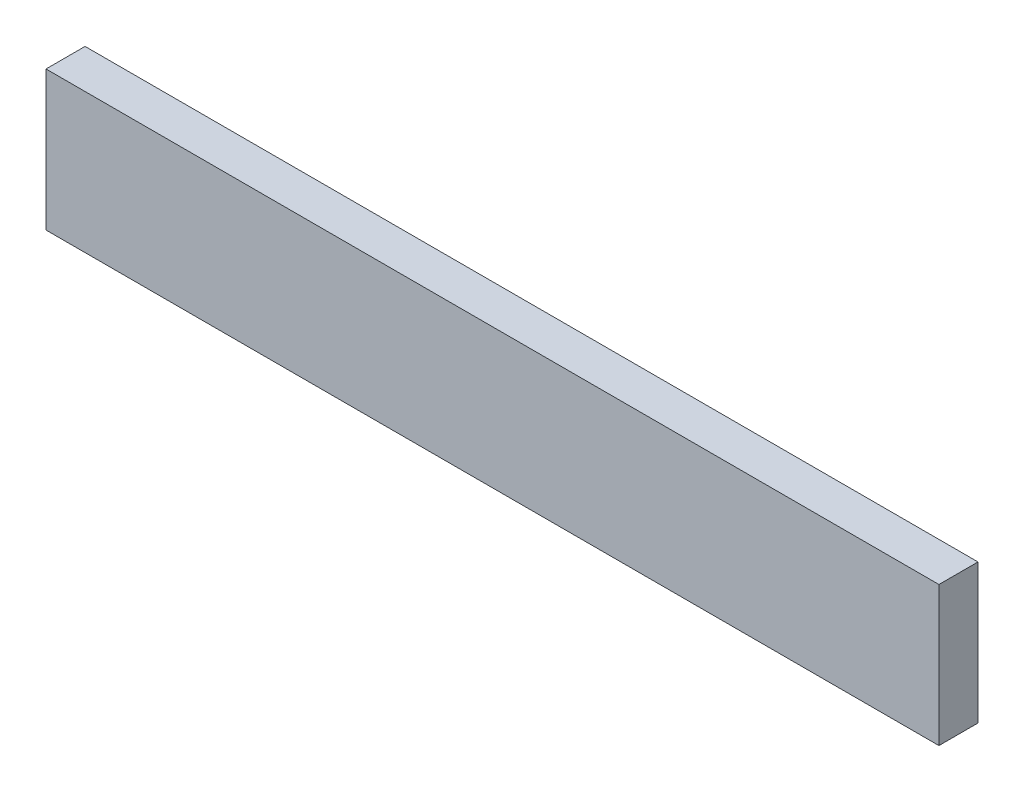
from build123d import *

# Parameters (mm, degrees)
SKETCH_1_W      = 160
SKETCH_1_H      = 25
EXTRUDE_1_DEPTH = 7


with BuildPart() as part:
    # 草图1 → 凸台-拉伸1 (new body)
    with BuildSketch(Plane.XY):
        Rectangle(SKETCH_1_W, SKETCH_1_H)
    extrude(amount=EXTRUDE_1_DEPTH)


solid = part.part
